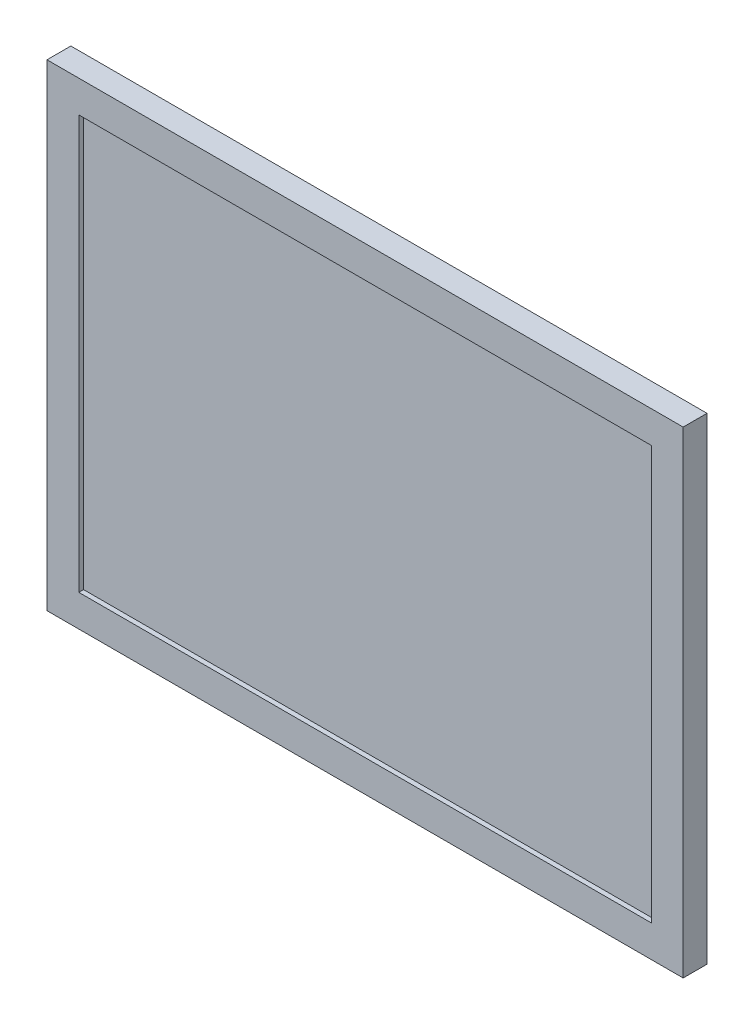
from build123d import *

# Parameters (mm, degrees)
EXTRUDE_1_DEPTH        = 200
EXTRUDE_1_DEPTH_BACK   = 200
SKETCH_6_W             = 360
SKETCH_6_H             = 260
CUT_EXTRUDE_1_DEPTH    = 3
CUT_EXTRUDE_2_REACH    = 370.623
HOLE_WIZARD_M4_1_D     = 3.3
HOLE_WIZARD_M4_1_DEPTH = 10.1
HOLE_WIZARD_M4_1_TIP   = 0.991420021


with BuildPart() as part:
    # 草图5 → 凸台-拉伸1 (new, two sides: drawn at the far end of the back side and taken through both)
    with BuildSketch(Plane.ZY.offset(-EXTRUDE_1_DEPTH_BACK)):
        Polygon((26.700089157, 410), (61.700089157, 510), (76.700089157, 510), (76.700089157, 210), (61.700089157, 210), (26.700089157, 290), align=None)
    extrude(amount=EXTRUDE_1_DEPTH + EXTRUDE_1_DEPTH_BACK)

    # 草图6 → 切除-拉伸1 (cut)
    with BuildSketch(Plane.XY.offset(76.700089157)):
        with Locations((0, 360)):
            Rectangle(SKETCH_6_W, SKETCH_6_H)
    extrude(amount=-CUT_EXTRUDE_1_DEPTH, mode=Mode.SUBTRACT)

    # 草图8 → 切除-拉伸2 (cut, up to next)
    with BuildSketch(Plane(origin=(0, 510, 0), x_dir=(1, 0, 0), z_dir=(0, 1, 0)), mode=Mode.PRIVATE) as cut_extrude_2_sk1:
        Polygon((-200, -61.700089157), (-200, -26.700089157), (-60, -26.700089157), align=None)
    cut_extrude_2_tool1 = extrude(cut_extrude_2_sk1.sketch, amount=-CUT_EXTRUDE_2_REACH, mode=Mode.PRIVATE) & part.part
    # 草图8 → 切除-拉伸2 (cut, up to next)
    with BuildSketch(Plane(origin=(0, 510, 0), x_dir=(1, 0, 0), z_dir=(0, 1, 0)), mode=Mode.PRIVATE) as cut_extrude_2_sk2:
        Polygon((60, -26.700089157), (200, -26.700089157), (200, -61.700089157), align=None)
    cut_extrude_2_tool2 = extrude(cut_extrude_2_sk2.sketch, amount=-CUT_EXTRUDE_2_REACH, mode=Mode.PRIVATE) & part.part
    add(cut_extrude_2_tool1.solids().sort_by_distance((-153.333333, 510, 38.366756))[0], mode=Mode.SUBTRACT)
    add(cut_extrude_2_tool2.solids().sort_by_distance((153.333333, 510, 38.366756))[0], mode=Mode.SUBTRACT)

    # M4 螺纹孔1
    with Locations(Plane(origin=(0, 0, 26.700089157), x_dir=(-1, 0, 0), z_dir=(0, 0, -1))):
        with Locations((-50, 400), (50, 400), (50, 300), (-50, 300)):
            Hole(HOLE_WIZARD_M4_1_D / 2, depth=HOLE_WIZARD_M4_1_DEPTH)
            with Locations((0, 0, -(HOLE_WIZARD_M4_1_DEPTH + HOLE_WIZARD_M4_1_TIP / 2))):  # 118° drill point
                Cone(0, HOLE_WIZARD_M4_1_D / 2, HOLE_WIZARD_M4_1_TIP, mode=Mode.SUBTRACT)


solid = part.part
